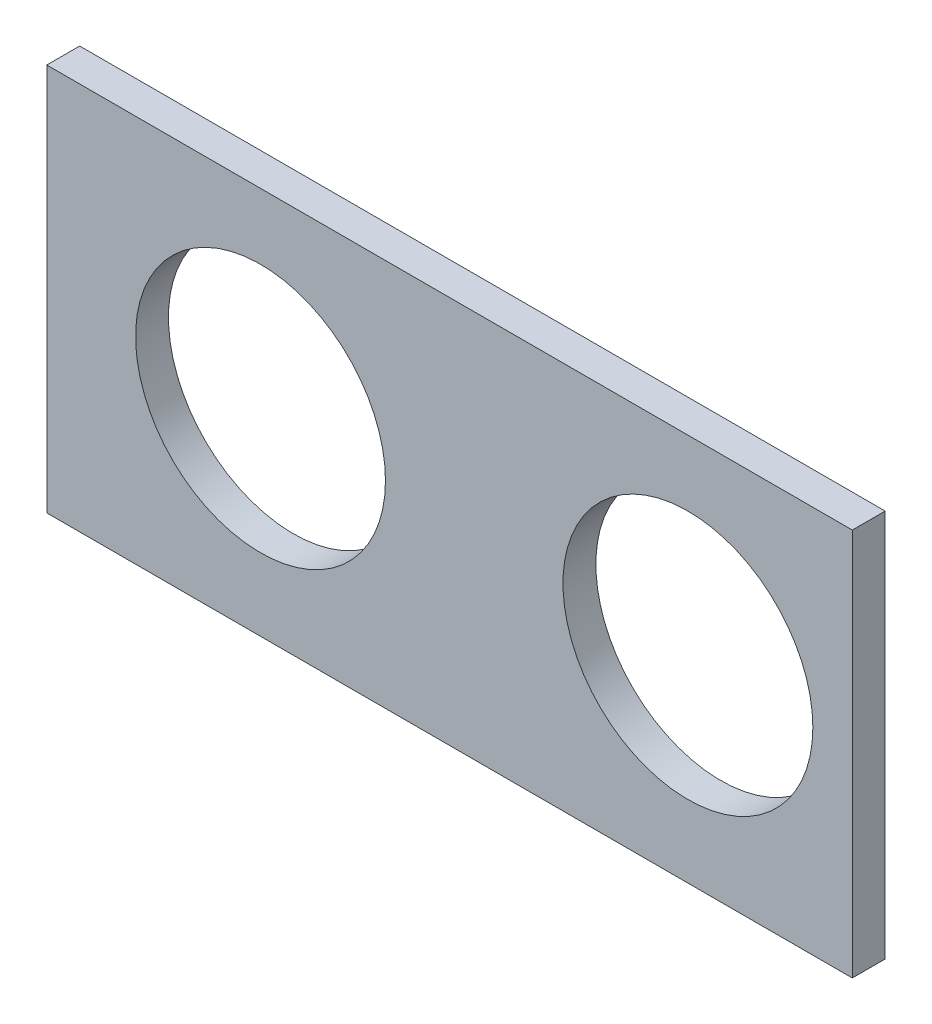
from build123d import *

# Parameters (mm, degrees)
SKETCH1_W           = 245
SKETCH1_H           = 118
SKETCH1_R           = 38
BOSS_EXTRUDE1_DEPTH = 10


with BuildPart() as part:
    # Sketch1 → Boss-Extrude1 (new body)
    with BuildSketch(Plane.XY):
        with Locations((122.5, 59)):
            Rectangle(SKETCH1_W, SKETCH1_H)
        with Locations((195, 60)):
            Circle(SKETCH1_R, mode=Mode.SUBTRACT)
        with Locations((65, 60)):
            Circle(SKETCH1_R, mode=Mode.SUBTRACT)
    extrude(amount=BOSS_EXTRUDE1_DEPTH)


solid = part.part
